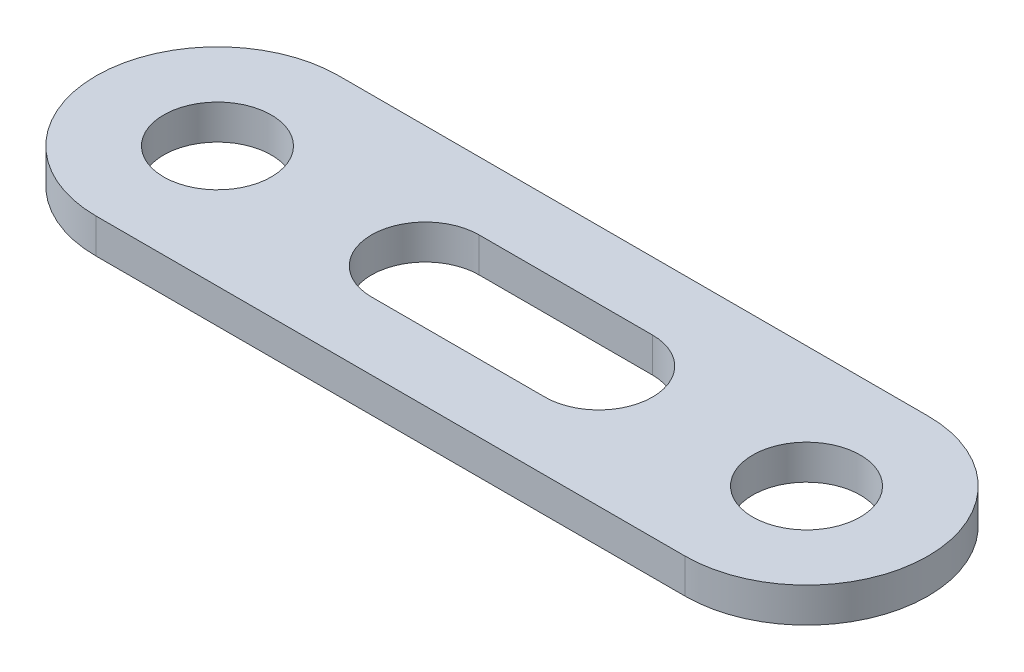
from build123d import *

# Parameters (mm, degrees)
SKETCH_1_R      = 1.55
EXTRUDE_1_DEPTH = 1


with BuildPart() as part:
    # 草图1 → 凸台-拉伸1 (new body)
    with BuildSketch(Plane(origin=(0, 0, 0), x_dir=(1, 0, 0), z_dir=(0, 1, 0))):
        with BuildLine():
            ThreePointArc((0, 3.5), (-3.5, 0), (0, -3.5))
            Line((0, -3.5), (16.98, -3.5))
            ThreePointArc((16.98, -3.5), (20.48, 0), (16.98, 3.5))
            Line((16.98, 3.5), (0, 3.5))
        make_face()
        with Locations(Location((0, 0, 0), (0, 0, 270))):
            Circle(SKETCH_1_R, mode=Mode.SUBTRACT)
        with BuildLine():
            ThreePointArc((10.99, 1.55), (12.54, 0), (10.99, -1.55))
            Line((10.99, -1.55), (5.99, -1.55))
            ThreePointArc((5.99, -1.55), (4.44, 0), (5.99, 1.55))
            Line((5.99, 1.55), (10.99, 1.55))
        make_face(mode=Mode.SUBTRACT)
        with Locations(Location((16.98, 0, 0), (0, 0, 270))):
            Circle(SKETCH_1_R, mode=Mode.SUBTRACT)
    extrude(amount=EXTRUDE_1_DEPTH)


solid = part.part
